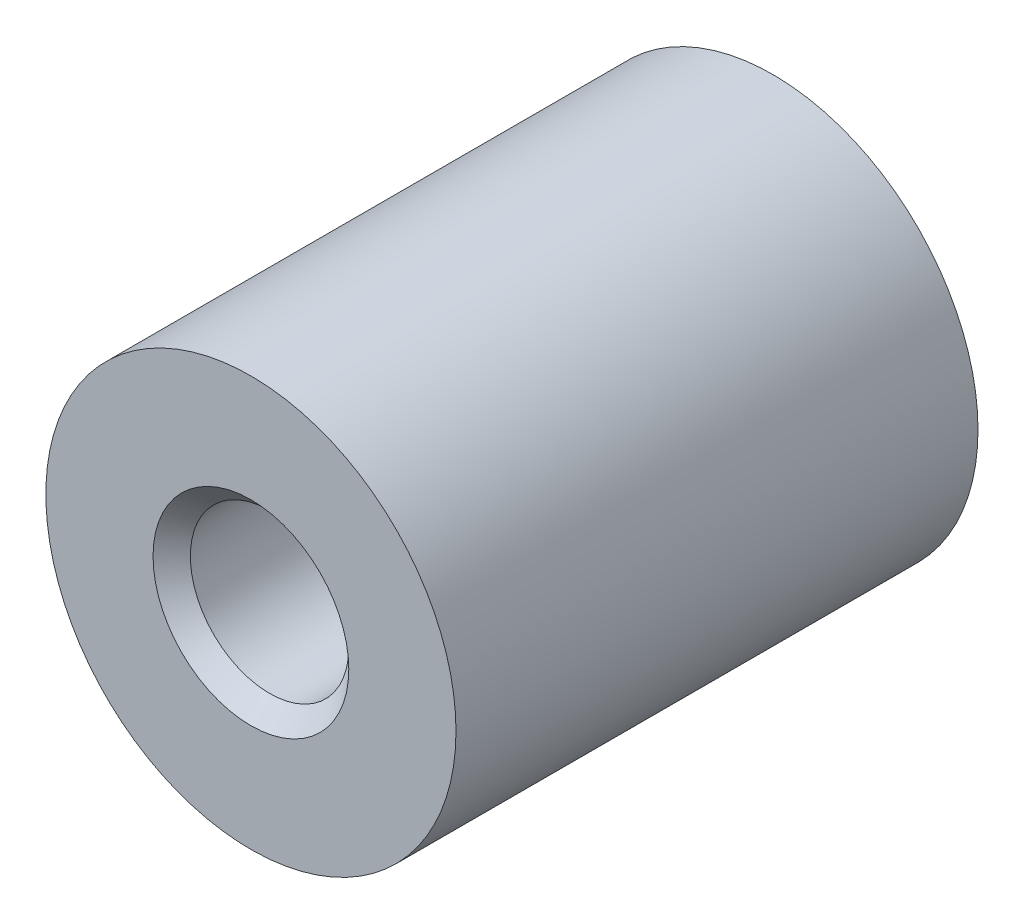
SolidWorks part; units mm, degrees
ref_plane "Front Plane" through (0, 0, 0) normal (0, 0, 1) x (1, 0, 0)
ref_plane "Top Plane" through (0, 0, 0) normal (0, 1, 0) x (1, 0, 0)
ref_plane "Right Plane" through (0, 0, 0) normal (1, 0, 0) x (0, 0, -1)
sketch "Sketch1" plane through (0, 0, 0) normal (0, 0, 1) x (1, 0, 0)
  circle A0 centre (0, 0) radius 11
extrude "Boss-Extrude1" add sketch "Sketch1" along normal blind 28
sketch "Sketch2" plane through (0, 0, 28) normal (0, 0, 1) x (1, 0, 0)
  circle A0 centre (0, 0) radius 4.25
extrude "Cut-Extrude1" cut sketch "Sketch2" against normal blind 38
sketch "Sketch3" plane through (0, 0, 28) normal (0, 0, 1) x (1, 0, 0)
  circle A0 centre (0, 0) radius 5
curve "Helix/Spiral1" pitch 1.5 height 18 turns 12
chamfer "Chamfer1" distance 1 angle 45 1 edges at (4.25, 0, 28)
